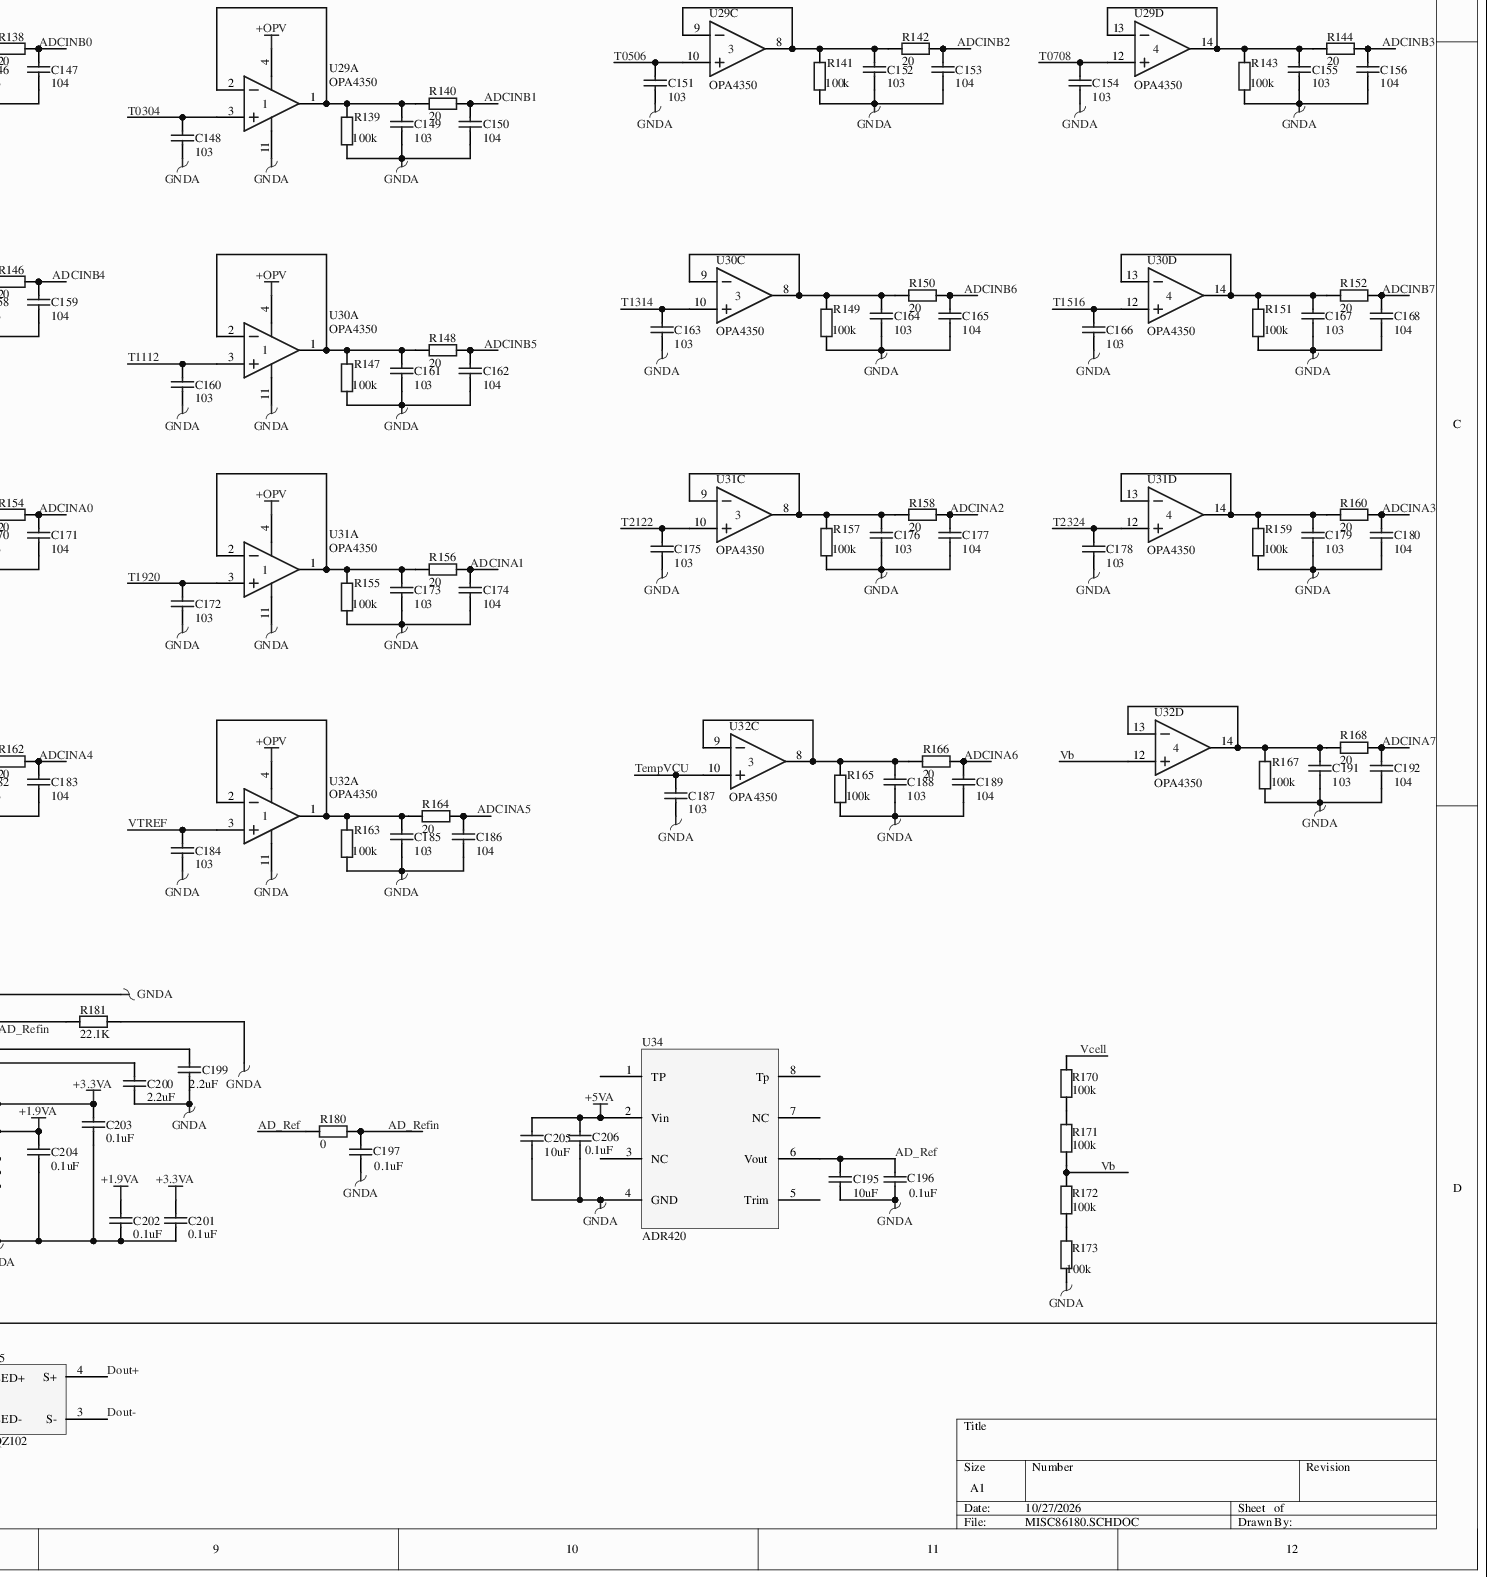
[diagram p0: MISC86180.SCHDOC, bottom right]
# Altium project MISC86180-9.PrjPCB (part 3 of 3)

## Sheet MISC86180.SCHDOC (continued)

### Nets
5VO1+: C9.1 C10.2 C64.2 C65.2 C66.2 C69.2 R23.2 U3.3(+Vout) U13.3(VCC) U15.1(ANODE1) U16.8(Vcc)
5VO1-: C9.2 C10.1 C58.1 C59.1 C60.1 C61.1 C62.1 C63.1 C64.1 C65.1 C66.1 C69.1 DZ1.2 DZ2.2 R20.1 U3.4(-Vout) U13.2(GND) U15.3(CATHODE2) U15.4(ANODE2) U16.5(GND)
+1.9VA: C46.2 C47.2 C48.2 C202.2 C204.2 L3.2 U9.31(VDD1A18) U9.59(VDD2A18)
+1.9VD: C13.1 C14.2 C30.2 C31.2 C32.2 C33.2 C34.2 C35.2 C36.2 C37.2 C38.2 C39.2 C40.2 C41.2 C42.2 L3.1 R3.2 U5.5(OUT) U5.6(OUT) U9.4(VDD(1V8).1) U9.15(VDD(1V8).2) U9.23(VDD(1V8).3) U9.29(VDD(1V8).4) U9.61(VDD(1V8).5) U9.101(VDD(1V8).6) U9.109(VDD(1V8).7) U9.117(VDD(1V8).8) U9.126(VDD(1V8).9) U9.139(VDD(1V8).10) U9.146(VDD(1V8).11) U9.154(VDD(1V8).12) U9.167(VDD(1V8).12)
+3.3VA: C15.1 C16.2 C125.2 C127.2 C201.2 C203.2 JC1.1 R131.1 R133.1 R136.1 U6.4(OUTPUT) U9.34(VDDA2(A3V3)) U9.45(VDDAIO(A3V3))
+3.3VD: C11.1 C12.2 C19.2 C20.2 C21.2 C22.2 C23.2 C24.2 C25.2 C26.2 C27.2 C28.2 C29.2 C68.2 J1.5 R1.1 R2.1 R6.1 R7.1 R8.2 R9.2 R10.2 R11.2 R12.2 R86.1 R88.1 R90.1 R92.1 R94.1 U4.4(OUTPUT) U5.3(IN) U5.4(IN) U8.5(VDD) U9.9(VDDIO(3V3).1) U9.71(VDDIO(3V3).2) U9.84(VDD3VFL.1) U9.93(VDDIO(3V3).3) U9.107(VDDIO(3V3).4) U9.121(VDDIO(3V3).5) U9.143(VDDIO(3V3).6) U9.159(VDDIO(3V3).7) U9.170(VDDIO(3V3).8) U16.1(ANODE1)
+3.3VD2: C17.1 C18.2 C81.1 C82.2 C83.2 C84.2 C85.2 C86.2 C87.2 C88.2 C89.2 C92.2 C93.2 C94.2 C95.2 J3.4 R84.1 R85.1 R95.1 U7.4(OUTPUT) U19.9(VCCIO1) U19.13(VCCINT_(3.3V_or_2.5V)) U19.31(VCCIO1) U19.45(VCCIO1) U19.59(VCCIO2) U19.63(VCCINT_(3.3V_or_2.5V)) U19.80(VCCIO2) U19.94(VCCIO2) U21.23(VCCB) U21.24(VCCB) U22.23(VCCB) U22.24(VCCB) U23.23(VCCB) U23.24(VCCB) U24.23(VCCB) U24.24(VCCB)
+5V: C6.1 C7.2 C57.2 C67.2 C90.2 C91.2 C96.2 C97.2 C98.2 C99.2 R21.2 U2.3(+Vout) U4.2(IN) U7.2(IN) U10.24(VDD) U15.8(Vcc) U20.24(VDD) U21.1(VCCA) U22.1(VCCA) U23.1(VCCA) U24.1(VCCA)
+5VA: C3.1 C4.2 C129.2 C130.2 C131.2 C140.2 C141.2 C142.2 C143.2 C144.2 C205.2 C206.2 U1.3(+Vout) U6.2(IN) U25.16(VCC) U26.16(VCC) U27.16(VCC) U28.16(VCC) U34.2(Vin)
+OPV: C132.2 C133.2 C134.2 C135.2 C136.2 C137.2 C138.2 C139.2 C208.2 C209.2 R136.2 U29.4(V+) U30.4(V+) U31.4(V+) U32.4(V+)
GNDA: C3.2 C4.1 C15.2 C16.1 C46.1 C47.1 C48.1 C100.1 C101.1 C102.1 C103.1 C104.1 C105.1 C106.1 C107.1 C108.1 C109.1 C110.1 C111.1 C112.1 C113.1 C114.1 C115.1 C116.1 C117.1 C118.1 C119.1 C120.1 C121.1 C122.1 C123.1 C124.1 C126.1 C128.1 C129.1 C130.1 C131.1 C132.1 C133.1 C134.1 C135.1 C136.1 C137.1 C138.1 C139.1 C140.1 C141.1 C142.1 C143.1 C144.1 C145.1 C146.1 C147.1 C148.1 C149.1 C150.1 C151.1 C152.1 C153.1 C154.1 C155.1 C156.1 C157.1 C158.1 C159.1 C160.1 C161.1 C162.1 C163.1 C164.1 C165.1 C166.1 C167.1 C168.1 C169.1 C170.1 C171.1 C172.1 C173.1 C174.1 C175.1 C176.1 C177.1 C178.1 C179.1 C180.1 C181.1 C182.1 C183.1 C184.1 C185.1 C186.1 C187.1 C188.1 C189.1 C191.1 C192.1 C195.1 C196.1 C197.1 C199.1 C200.1 C201.1 C202.1 C203.1 C204.1 C205.1 C206.1 C208.1 C209.1 L2.2 R105.1 R106.2 R107.2 R108.2 R109.2 R110.2 R111.2 R112.2 R113.2 R114.2 R115.2 R116.2 R117.2 R118.2 R119.2 R120.2 R121.2 R122.2 R123.2 R124.2 R125.2 R126.2 R127.2 R128.2 R129.2 R130.2 R132.2 R134.2 R137.1 R139.1 R141.1 R143.1 R145.1 R147.1 R149.1 R151.1 R153.1 R155.1 R157.1 R159.1 R161.1 R163.1 R165.1 R167.1 R173.2 R181.2 S1.5(S2_2) S2.5(S2_2) S3.5(S2_2) S4.5(S2_2) S5.5(S2_2) S6.5(S2_2) S7.5(S2_2) S8.5(S2_2) S9.5(S2_2) S10.5(S2_2) S11.5(S2_2) S12.5(S2_2) S13.5(S2_2) S14.5(S2_2) S15.5(S2_2) S16.5(S2_2) S17.5(S2_2) S18.5(S2_2) S19.5(S2_2) S20.5(S2_2) S21.5(S2_2) S22.5(S2_2) S23.5(S2_2) S24.5(S2_2) U1.4(-Vout) U6.1(~{EN}) U6.3(GND) U9.32(VSS1AGND) U9.33(VSSA2(AGND)) U9.43(ADCLO) U9.44(VSSAIO(AGND)) U9.58(VSS2AGND) U25.6(~{EN}) U25.8(GND) U26.6(~{EN}) U26.8(GND) U27.6(~{EN}) U27.8(GND) U28.6(~{EN}) U28.8(GND) U29.11(V-) U30.11(V-) U31.11(V-) U32.11(V-) U34.4(GND)
GNDD: C6.2 C7.1 C11.2 C12.1 C13.2 C14.1 C17.2 C18.1 C19.1 C20.1 C21.1 C22.1 C23.1 C24.1 C25.1 C26.1 C27.1 C28.1 C29.1 C30.1 C31.1 C32.1 C33.1 C34.1 C35.1 C36.1 C37.1 C38.1 C39.1 C40.1 C41.1 C42.1 C52.1 C53.1 C54.1 C55.1 C56.1 C57.1 C67.1 C68.1 C81.2 C82.1 C83.1 C84.1 C85.1 C86.1 C87.1 C88.1 C89.1 C90.1 C91.1 C92.1 C93.1 C94.1 C95.1 C96.1 C97.1 C98.1 C99.1 D1.2(K) D2.2(K) D3.2(K) D4.2(K) D5.2(K) D6.2(K) D7.2(K) D8.2(K) D9.2(K) D10.2(K) J1.4 J1.6 J1.8 J1.10 J1.12 J3.2 J3.10 L2.1 R4.1 R5.1 R14.1 R83.1 R87.2 R89.2 R91.2 R93.2 S1.2(LED1-) S1.4(LED2-) S2.2(LED1-) S2.4(LED2-) S3.2(LED1-) S3.4(LED2-) S4.2(LED1-) S4.4(LED2-) S5.2(LED1-) S5.4(LED2-) S6.2(LED1-) S6.4(LED2-) S7.2(LED1-) S7.4(LED2-) S8.2(LED1-) S8.4(LED2-) S9.2(LED1-) S9.4(LED2-) S10.2(LED1-) S10.4(LED2-) S11.2(LED1-) S11.4(LED2-) S12.2(LED1-) S12.4(LED2-) S13.2(LED1-) S13.4(LED2-) S14.2(LED1-) S14.4(LED2-) S15.2(LED1-) S15.4(LED2-) S16.2(LED1-) S16.4(LED2-) S17.2(LED1-) S17.4(LED2-) S18.2(LED1-) S18.4(LED2-) S19.2(LED1-) S19.4(LED2-) S20.2(LED1-) S20.4(LED2-) S21.2(LED1-) S21.4(LED2-) S22.2(LED1-) S22.4(LED2-) S23.2(LED1-) S23.4(LED2-) S24.2(LED1-) S24.4(LED2-) SW1.2 U2.4(-Vout) U4.1(~{EN}) U4.3(GND) U5.1(GND) U7.1(~{EN}) U7.3(GND) U8.2(GND) U9.3(VSS.1) U9.8(VSS.2) U9.14(VSS.3) U9.22(VSS.4) U9.30(VSS.5) U9.60(VSS.6) U9.70(VSS.7) U9.83(VSS.8) U9.92(VSS.9) U9.103(VSS.10) U9.105(XCLKIN) U9.106(VSS.11) U9.108(VSS.12) U9.118(VSS.13) U9.120(VSS.14) U9.125(VSS.15) U9.140(VSS.16) U9.144(VSS.17) U9.147(VSS.18) U9.155(VSS.19) U9.160(VSS.19) U9.166(VSS.20) U9.171(VSS.21) U10.1(~{OE}1) U10.12(GND) U10.13(~{OE}2) U15.5(GND) U16.3(CATHODE2) U16.4(ANODE2) U19.10(GNDIO) U19.11(GNDINT) U19.32(GNDIO) U19.46(GNDIO) U19.50(IO) U19.60(GNDIO) U19.65(GNDINT) U19.79(GNDIO) U19.93(GNDIO) U20.1(~{OE}1) U20.12(GND) U20.13(~{OE}2) U21.2(DIR) U21.11(GND) U21.12(GND) U21.13(GND) U21.22(~{OE}) U22.2(DIR) U22.11(GND) U22.12(GND) U22.13(GND) U22.22(~{OE}) U23.2(DIR) U23.11(GND) U23.12(GND) U23.13(GND) U23.22(~{OE}) U24.2(DIR) U24.11(GND) U24.12(GND) U24.13(GND) U24.22(~{OE}) U35.1(LED-) Y1.3
12V+: B1.2(CB) C2.1 C5.1 C8.1 U1.1(+Vin) U2.1(+Vin) U3.1(+Vin)
12V-: B1.4(CG) B1.5(CG) B1.6(CG) C2.2 C5.2 C8.2 U1.2(-Vin) U2.2(-Vin) U3.2(-Vin)
12Vin+: F49.2 JC2.26 JC2.34
12Vin-: B1.3(PSG) C1.2 JC2.25 JC2.33 TVS1.1
A1_12: R12.1 U9.169(XA12)
A1_13: R11.1 U9.172(XA13)
A1_14: R10.1 U9.173(XA14)
A1_15: R9.1 U9.174(XA15)
AD_Ref: C195.2 C196.2 R180.2 U34.6(Vout)
AD_Refin: C197.2 R180.1 U9.54(ADCREFIN)
ADCINA0: C171.2 R154.1 U9.42(ADCINA0)
ADCINA1: C174.2 R156.1 U9.41(ADCINA1)
ADCINA2: C177.2 R158.1 U9.40(ADCINA2)
ADCINA3: C180.2 R160.1 U9.39(ADCINA3)
ADCINA4: C183.2 R162.1 U9.38(ADCINA4)
ADCINA5: C186.2 R164.1 U9.37(ADCINA5)
ADCINA6: C189.2 R166.1 U9.36(ADCINA6)
ADCINA7: C192.2 R168.1 U9.35(ADCINA7)
ADCINB0: C147.2 R138.1 U9.46(ADCINB0)
ADCINB1: C150.2 R140.1 U9.47(ADCINB1)
ADCINB2: C153.2 R142.1 U9.48(ADCINB2)
ADCINB3: C156.2 R144.1 U9.49(ADCINB3)
ADCINB4: C159.2 R146.1 U9.50(ADCINB4)
ADCINB5: C162.2 R148.1 U9.51(ADCINB5)
ADCINB6: C165.2 R150.1 U9.52(ADCINB6)
ADCINB7: C168.2 R152.1 U9.53(ADCINB7)
BAT1: F1.1 JC1.24
BAT2: F2.1 F3.1 JC1.32
BAT3: F4.1 F5.1 JC1.25
BAT4: F6.1 F7.1 JC1.33
BAT5: F8.1 F9.1 JC1.26
BAT6: F10.1 F11.1 JC1.34
BAT7: F12.1 F13.1 JC1.27
BAT8: F14.1 F15.1 JC1.35
BAT9: F16.1 F17.1 JC1.28
BAT10: F18.1 F19.1 JC1.36
BAT11: F20.1 F21.1 JC2.3
BAT12: F22.1 F23.1 JC2.13
BAT13: F24.1 F25.1 JC2.4
BAT14: F26.1 F27.1 JC2.14
BAT15: F28.1 F29.1 JC2.5
BAT16: F30.1 F31.1 JC2.15
BAT17: F32.1 F33.1 JC2.6
BAT18: F34.1 F35.1 JC2.16
BAT19: F36.1 F37.1 JC2.7
BAT20: F38.1 F39.1 JC2.17
BAT21: F40.1 F41.1 JC2.8
BAT22: F42.1 F43.1 JC2.18
BAT23: F44.1 F45.1 JC2.9
BAT24: F46.1 F47.1 JC2.19
BAT25: F48.1 JC2.10
CAN1H: C60.2 DZ1.1 JC2.23 JC2.31 R17.2 U11.4
CAN1HIN: C58.2 U11.1 U13.7(CANH)
CAN1L: C61.2 DZ2.1 JC2.22 JC2.30 R18.1 U11.3
CAN1LIN: C59.2 U11.2 U13.6(CANL)
CAN1RX: R22.2 U13.4(R)
CAN1S: JC2.21 JC2.29 R19.2
CAN1TX: R23.1 U13.1(D) U16.7(Vo1)
CANAR: R13.1 R14.2 U10.9(1B4)
CANARR: R13.2 R21.1 U15.7(Vo1)
CANARX: U9.62(GPIO18/SPICLKA/SCITXDB/CANRXA) U10.8(1A4)
CANAT: R24.2 U10.5(1B2)
CANATX: U9.63(GPIO19/SPISTEAn/SCIRXDB/CANTXA) U10.4(1A2)
CI1: U19.69(IO) U20.2(1B1)
CI2: U19.70(IO) U20.10(1B5)
CI3: U19.71(IO) U20.5(1B2)
CI4: U19.72(IO) U20.16(2B2)
CI5: U19.73(IO) U20.6(1B3)
CI6: U19.74(IO) U20.15(2B1)
CI7: U19.75(IO) U20.9(1B4)
CI9: R96.1 U20.23(2B5)
CI10: R97.1 U20.20(2B4)
CO1: U19.66(IO) U22.16(B6)
CO2: U19.64(IO/GCLK3) U22.17(B5)
CO3: U19.62(IO/GCLK2) U22.18(B4)
CO4: U19.61(IO) U22.19(B3)
CO5: U19.57(IO) U22.21(B1)
CO6: U19.58(IO) U22.20(B2)
CO7: U19.51(IO) U21.14(B8)
CO8: U19.52(IO) U21.15(B7)
CO9: U19.53(IO) U21.16(B6)
CO10: U19.54(IO) U21.17(B5)
CO11: U19.55(IO) U21.18(B4)
CO12: U19.56(IO) U21.19(B3)
CO13: U19.7(IO) U23.19(B3)
CO14: U19.8(IO) U23.18(B4)
CO15: U19.12(IO/GCLK0) U23.17(B5)
CO16: U19.14(IO/GCLK1) U23.16(B6)
CO17: U19.15(IO) U23.15(B7)
CO18: U19.16(IO) U23.14(B8)
CO19: U19.6(IO) U24.19(B3)
CO20: U19.5(IO) U24.18(B4)
CO21: U19.4(IO) U24.17(B5)
CO22: U19.3(IO) U24.16(B6)
CO23: U19.2(IO) U24.15(B7)
CO24: U19.1(IO) U24.14(B8)
CO25: U19.67(IO) U22.15(B7)
CO26: U19.68(IO) U22.14(B8)
CT1: R33.2 R34.2 U22.8(A6)
CT2: R35.2 R36.2 U22.7(A5)
CT3: R37.2 R38.2 U22.6(A4)
CT4: R41.2 R42.2 U22.5(A3)
CT5: R43.2 R44.2 U22.3(A1)
CT6: R45.2 R46.2 U22.4(A2)
CT7: R47.2 R48.2 U21.10(A8)
CT8: R49.2 R50.2 U21.9(A7)
CT9: R51.2 R52.2 U21.8(A6)
CT10: R53.2 R54.2 U21.7(A5)
CT11: R55.2 R56.2 U21.6(A4)
CT12: R57.2 R58.2 U21.5(A3)
CT13: R59.2 R60.2 U23.5(A3)
CT14: R61.2 R62.2 U23.6(A4)
CT15: R63.2 R64.2 U23.7(A5)
CT16: R65.2 R66.2 U23.8(A6)
CT17: R67.2 R68.2 U23.9(A7)
CT18: R69.2 R70.2 U23.10(A8)
CT19: R71.2 R72.2 U24.5(A3)
CT20: R73.2 R74.2 U24.6(A4)
CT21: R75.2 R76.2 U24.7(A5)
CT22: R77.2 R78.2 U24.8(A6)
CT23: R79.2 R80.2 U24.9(A7)
CT24: R81.2 R82.2 U24.10(A8)
CT25: L1.1 U22.10(A8)
CT26: R104.2 U22.9(A7)
CTCK: J3.1 R83.2 U19.24(TCK)
CTDI: J3.9 R85.2 U19.23(TDI)
CTDO: J3.3 U19.25(TDO)
CTMS: J3.5 R84.2 U19.22(TMS)
CTOUT25: L1.2 R105.2 U25.9(C) U25.10(B) U25.11(A) U26.9(C) U26.10(B) U26.11(A) U27.9(C) U27.10(B) U27.11(A) U28.9(C) U28.10(B) U28.11(A)
Dout+: JC2.24 U35.4(S+)
Dout-: JC2.32 U35.3(S-)
EMU0: C53.2 J1.13 R6.2 U9.85(EMU0)
EMU1: C54.2 J1.14 R7.2 U9.86(EMU1)
GPIO0: U9.5(GPIO0/EPWM1A) U20.3(1A1)
GPIO1: U9.6(GPIO1/EPWM1B/ECAP6/MFSRB) U20.11(1A5)
GPIO2: U9.7(GPIO2/EPWM2A) U20.4(1A2)
GPIO3: U9.10(GPIO3/EPWM2B/ECAP5/MCLKRB) U20.17(2A2)
GPIO4: U9.11(GPIO4/EPWM3A) U20.7(1A3)
GPIO5: U9.12(GPIO5/EPWM3B/MFSRA/ECAP1) U20.14(2A1)
GPIO6: U9.13(GPIO6/EPWM4A/EPWMSYNCI/EPWMSYNCO) U20.8(1A4)
GPIO8: U9.17(GPIO8/EPWM5A/CANTXB/ADCSOCAOn) U20.22(2A5)
GPIO9: U9.18(GPIO9/EPWM5B/SCITXDB/ECAP3) U20.21(2A4)
GPIO10: R86.2 R87.1 U9.19(GPIO10/EPWM6A/CANRXB/ADCSOCBOn)
GPIO11: R88.2 R89.1 U9.20(GPIO11/EPWM6B/SCIRXDB/ECAP4)
GPIO12: R90.2 R91.1 U9.21(GPIO12/TZ1n/CANTXB/MDXB)
GPIO13: R92.2 R93.1 U9.24(GPIO13/TZ2n/CANRXB/MDRB)
LED1: R98.1 U19.76(IO)
LED2: R99.1 U19.81(IO)
LED3: R100.1 U19.82(IO)
LED4: R101.1 U19.88(IO)
LED5: R102.1 U19.89(IO)
LED6: R103.1 U19.97(IO)
~{MR}: SW1.1 U8.3(~{MR})
~{PG}: R1.2 U4.5(FB/~{PG}) U5.2(~{EN})
~{RESET}: R2.2 U8.1(~{RESE}T) U9.80(~{XRS})
T0102: C145.2 U25.14(X) U29.5(IN+)
T0304: C148.2 U25.15(Y) U29.3(IN+)
T0506: C151.2 U25.4(Z) U29.10(IN+)
T0708: C154.2 U28.14(X) U29.12(IN+)
T0910: C157.2 U28.15(Y) U30.5(IN+)
T1112: C160.2 U28.4(Z) U30.3(IN+)
T1314: C163.2 U27.15(Y) U30.10(IN+)
T1516: C166.2 U27.4(Z) U30.12(IN+)
T1718: C169.2 U27.14(X) U31.5(IN+)
T1920: C172.2 U26.14(X) U31.3(IN+)
T2122: C175.2 U26.15(Y) U31.10(IN+)
T2324: C178.2 U26.4(Z) U31.12(IN+)
~{TRST}: C52.2 J1.2 R5.2 U9.78(~{TRST})
TCK: J1.9 J1.11 U9.87(TCK)
TDI: J1.3 U9.76(TDI)
TDO: J1.7 U9.77(TDO)
Temp1: C100.2 JC1.11 R106.1 U25.12(X0)
Temp2: C101.2 JC1.2 R107.1 U25.13(X1)
Temp3: C102.2 JC1.12 R108.1 U25.2(Y0)
Temp4: C103.2 JC1.3 R109.1 U25.1(Y1)
Temp5: C104.2 JC1.13 R110.1 U25.5(Z0)
Temp6: C105.2 JC1.4 R111.1 U25.3(Z1)
Temp7: C106.2 JC1.14 R112.1 U28.12(X0)
Temp8: C107.2 JC1.5 R113.1 U28.13(X1)
Temp9: C108.2 JC1.15 R114.1 U28.2(Y0)
Temp10: C109.2 JC1.6 R115.1 U28.1(Y1)
Temp11: C110.2 JC1.16 R116.1 U28.5(Z0)
Temp12: C111.2 JC1.7 R117.1 U28.3(Z1)
Temp13: C112.2 JC1.17 R118.1 U27.2(Y0)
Temp14: C113.2 JC1.8 R119.1 U27.1(Y1)
Temp15: C114.2 JC1.18 R120.1 U27.5(Z0)
Temp16: C115.2 JC1.9 R121.1 U27.3(Z1)
Temp17: C116.2 JC1.19 R122.1 U27.12(X0)
Temp18: C117.2 JC1.10 R123.1 U27.13(X1)
Temp19: C118.2 JC1.20 R124.1 U26.12(X0)
Temp20: C119.2 JC1.21 R125.1 U26.13(X1)
Temp21: C120.2 JC1.29 R126.1 U26.2(Y0)
Temp22: C121.2 JC1.22 R127.1 U26.1(Y1)
Temp23: C122.2 JC1.30 R128.1 U26.5(Z0)
Temp24: C123.2 JC1.23 R129.1 U26.3(Z1)
Temp25: C124.2 C181.2 JC1.31 R130.1 U32.5(IN+)
TempVCU: C127.1 C128.2 C187.2 R133.2 R134.1 U32.10(IN+)
TMS: J1.1 U9.79(TMS)
Vb: R171.2 R172.1 U32.12(IN+)
Vcell: R170.1 S1.7(S1_2) S2.7(S1_2) S3.7(S1_2) S4.7(S1_2) S5.7(S1_2) S6.7(S1_2) S7.7(S1_2) S8.7(S1_2) S9.7(S1_2) S10.7(S1_2) S11.7(S1_2) S12.7(S1_2) S13.7(S1_2) S14.7(S1_2) S15.7(S1_2) S16.7(S1_2) S17.7(S1_2) S18.7(S1_2) S19.7(S1_2) S20.7(S1_2) S21.7(S1_2) S22.7(S1_2) S23.7(S1_2) S24.7(S1_2)
VTREF: C125.1 C126.2 C184.2 R131.2 R132.1 U32.3(IN+)
NetB1_1: B1.1(B) C1.1 F49.1 TVS1.2
NetC55_2: C55.2 U9.102(X2) Y1.1
NetC56_2: C56.2 U9.104(X1) Y1.2
NetC62_2: C62.2 R17.1 R18.2
NetC63_2: C63.2 R19.1
NetC146_2: C146.2 R137.2 R138.2 U29.6(IN-) U29.7(OUT)
NetC149_2: C149.2 R139.2 R140.2 U29.1(OUT) U29.2(IN-)
NetC152_2: C152.2 R141.2 R142.2 U29.8(OUT) U29.9(IN-)
NetC155_2: C155.2 R143.2 R144.2 U29.13(IN-) U29.14(OUT)
NetC158_2: C158.2 R145.2 R146.2 U30.6(IN-) U30.7(OUT)
NetC161_2: C161.2 R147.2 R148.2 U30.1(OUT) U30.2(IN-)
NetC164_2: C164.2 R149.2 R150.2 U30.8(OUT) U30.9(IN-)
NetC167_2: C167.2 R151.2 R152.2 U30.13(IN-) U30.14(OUT)
NetC170_2: C170.2 R153.2 R154.2 U31.6(IN-) U31.7(OUT)
NetC173_2: C173.2 R155.2 R156.2 U31.1(OUT) U31.2(IN-)
NetC176_2: C176.2 R157.2 R158.2 U31.8(OUT) U31.9(IN-)
NetC179_2: C179.2 R159.2 R160.2 U31.13(IN-) U31.14(OUT)
NetC182_2: C182.2 R161.2 R162.2 U32.6(IN-) U32.7(OUT)
NetC185_2: C185.2 R163.2 R164.2 U32.1(OUT) U32.2(IN-)
NetC188_2: C188.2 R165.2 R166.2 U32.8(OUT) U32.9(IN-)
NetC191_2: C191.2 R167.2 R168.2 U32.13(IN-) U32.14(OUT)
NetC199_2: C199.2 U9.56(ADCREFP)
NetC200_2: C200.2 U9.55(ADCREFM)
NetD1_1: D1.1(A) R94.2
NetD2_1: D2.1(A) R95.2
NetD3_1: D3.1(A) R96.2
NetD4_1: D4.1(A) R97.2
NetD5_1: D5.1(A) R98.2
NetD6_1: D6.1(A) R99.2
NetD7_1: D7.1(A) R100.2
NetD8_1: D8.1(A) R101.2
NetD9_1: D9.1(A) R102.2
NetD10_1: D10.1(A) R103.2
NetF1_2: F1.2 S1.8(S1_1)
NetF2_2: F2.2 S1.6(S2_1)
NetF3_2: F3.2 S2.8(S1_1)
NetF4_2: F4.2 S2.6(S2_1)
NetF5_2: F5.2 S3.8(S1_1)
NetF6_2: F6.2 S3.6(S2_1)
NetF7_2: F7.2 S4.8(S1_1)
NetF8_2: F8.2 S4.6(S2_1)
NetF9_2: F9.2 S5.8(S1_1)
NetF10_2: F10.2 S5.6(S2_1)
NetF11_2: F11.2 S6.8(S1_1)
NetF12_2: F12.2 S6.6(S2_1)
NetF13_2: F13.2 S7.8(S1_1)
NetF14_2: F14.2 S7.6(S2_1)
NetF15_2: F15.2 S8.8(S1_1)
NetF16_2: F16.2 S8.6(S2_1)
NetF17_2: F17.2 S9.8(S1_1)
NetF18_2: F18.2 S9.6(S2_1)
NetF19_2: F19.2 S10.8(S1_1)
NetF20_2: F20.2 S10.6(S2_1)
NetF21_2: F21.2 S11.8(S1_1)
NetF22_2: F22.2 S11.6(S2_1)
NetF23_2: F23.2 S12.8(S1_1)
NetF24_2: F24.2 S12.6(S2_1)
NetF25_2: F25.2 S13.8(S1_1)
NetF26_2: F26.2 S13.6(S2_1)
NetF27_2: F27.2 S14.8(S1_1)
NetF28_2: F28.2 S14.6(S2_1)
NetF29_2: F29.2 S15.8(S1_1)
NetF30_2: F30.2 S15.6(S2_1)
NetF31_2: F31.2 S16.8(S1_1)
NetF32_2: F32.2 S16.6(S2_1)
NetF33_2: F33.2 S17.8(S1_1)
NetF34_2: F34.2 S17.6(S2_1)
NetF35_2: F35.2 S18.8(S1_1)
NetF36_2: F36.2 S18.6(S2_1)
NetF37_2: F37.2 S19.8(S1_1)
NetF38_2: F38.2 S19.6(S2_1)
NetF39_2: F39.2 S20.8(S1_1)
NetF40_2: F40.2 S20.6(S2_1)
NetF41_2: F41.2 S21.8(S1_1)
NetF42_2: F42.2 S21.6(S2_1)
NetF43_2: F43.2 S22.8(S1_1)
NetF44_2: F44.2 S22.6(S2_1)
NetF45_2: F45.2 S23.8(S1_1)
NetF46_2: F46.2 S23.6(S2_1)
NetF47_2: F47.2 S24.8(S1_1)
NetF48_2: F48.2 S24.6(S2_1)
NetJ2_1: J2.1 U9.99(GPIO57/SPISTEAn/XD22)
NetJ2_2: J2.2 U9.98(GPIO56/SPICLKA/XD23)
NetJ2_3: J2.3 U9.97(GPIO55/SPISOMIA/XD24)
NetJ2_4: J2.4 U9.96(GPIO54/SPISIMOA/XD25)
NetR3_1: R3.1 R4.2 U5.7(FB/NC)
NetR8_1: R8.1 U9.142(XREADY)
NetR20_2: R20.2 U13.8(RS)
NetR22_1: R22.1 U15.2(CATHODE1)
NetR24_1: R24.1 U16.2(CATHODE1)
NetR33_1: R33.1 S1.1(LED1+)
NetR34_1: R34.1 S1.3(LED2+)
NetR35_1: R35.1 S2.1(LED1+)
NetR36_1: R36.1 S2.3(LED2+)
NetR37_1: R37.1 S3.1(LED1+)
NetR38_1: R38.1 S3.3(LED2+)
NetR41_1: R41.1 S4.1(LED1+)
NetR42_1: R42.1 S4.3(LED2+)
NetR43_1: R43.1 S5.1(LED1+)
NetR44_1: R44.1 S5.3(LED2+)
NetR45_1: R45.1 S6.1(LED1+)
NetR46_1: R46.1 S6.3(LED2+)
NetR47_1: R47.1 S7.1(LED1+)
NetR48_1: R48.1 S7.3(LED2+)
NetR49_1: R49.1 S8.1(LED1+)
NetR50_1: R50.1 S8.3(LED2+)
NetR51_1: R51.1 S9.1(LED1+)
NetR52_1: R52.1 S9.3(LED2+)
NetR53_1: R53.1 S10.1(LED1+)
NetR54_1: R54.1 S10.3(LED2+)
NetR55_1: R55.1 S11.1(LED1+)
NetR56_1: R56.1 S11.3(LED2+)
NetR57_1: R57.1 S12.1(LED1+)
NetR58_1: R58.1 S12.3(LED2+)
NetR59_1: R59.1 S13.1(LED1+)
NetR60_1: R60.1 S13.3(LED2+)
NetR61_1: R61.1 S14.1(LED1+)
NetR62_1: R62.1 S14.3(LED2+)
NetR63_1: R63.1 S15.1(LED1+)
NetR64_1: R64.1 S15.3(LED2+)
NetR65_1: R65.1 S16.1(LED1+)
NetR66_1: R66.1 S16.3(LED2+)
NetR67_1: R67.1 S17.1(LED1+)
NetR68_1: R68.1 S17.3(LED2+)
NetR69_1: R69.1 S18.1(LED1+)
NetR70_1: R70.1 S18.3(LED2+)
NetR71_1: R71.1 S19.1(LED1+)
NetR72_1: R72.1 S19.3(LED2+)
NetR73_1: R73.1 S20.1(LED1+)
NetR74_1: R74.1 S20.3(LED2+)
NetR75_1: R75.1 S21.1(LED1+)
NetR76_1: R76.1 S21.3(LED2+)
NetR77_1: R77.1 S22.1(LED1+)
NetR78_1: R78.1 S22.3(LED2+)
NetR79_1: R79.1 S23.1(LED1+)
NetR80_1: R80.1 S23.3(LED2+)
NetR81_1: R81.1 S24.1(LED1+)
NetR82_1: R82.1 S24.3(LED2+)
NetR104_1: R104.1 U35.2(LED+)
NetR170_2: R170.2 R171.1
NetR172_2: R172.2 R173.1
NetR181_1: R181.1 U9.57(ADCRESEXT)

Not connected (* = marked no-connect by the designer): J3 6 7 8; JC2 20; U5 8(PG)*; U6 5(FB/~{PG}); U7 5(FB/~{PG}); U8 4(WDI)*; U9 1(XA18)* 2(XA19)* 16(GPIO7/EPWM4B/MCLKRA/ECAP2) 25(~{XHOLD})* 26(~{XHOLDA})* 27(GPIO16/SPISIMOA/CANTXB/TZ5n)* 28(GPIO17/SPISOMIA/CANRXB/TZ6n)* 64(GPIO20/EQEP1A/MDXA/CANTXB)* 65(GPIO21/EQEP1B/MDRA/CANRXB)* 66(GPIO22/EQEP1S/MCLKXA/SCITXDB)* 67(GPIO23/EQEP1I/MFSXA/SCIRXDB)* 68(GPIO24/ECAP1/EQEP2A/MDXB)* 69(GPIO25/ECAP2/EQEP2B/MDRB)* 72(GPIO26/ECAP3/EQEP2I/MCLKXB)* 73(GPIO27/ECAP4/EQEP2S/MFSXB)* 74(GPIO32/SDAA/EPWMSYNCI/ADCSOCAOn)* 75(GPIO33/SCLA/EPWMSYNCO/ADCSOCBOn)* 81((NC)_TEST1)* 82((NC)_TEST2)* 88(GPIO48/ECAP5/XD31)* 89(GPIO49/ECAP6/XD30)* 90(GPIO50/EQEP1A/XD29)* 91(GPIO51/EQEP1B/XD28)* 94(GPIO52/EQEP1S/XD27)* 95(GPIO53/EQEP1I/XD26)* 100(GPIO58/MCLKRA/XD21)* 110(GPIO59/MFSRA/XD20)* 111(GPIO60/MCLKRB/XD19)* 112(GPIO61/MFSRB/XD18)* 113(GPIO62/SCIRXDC/XD17)* 114(GPIO63/SCITXDC/XD16)* 115(XD15)* 116(XD14)* 119(XD13)* 122(XD12)* 123(XD11)* 124(XD10)* 127(XD9)* 128(XD8)* 129(XD7)* 130(XD6)* 131(XD5)* 132(XD4)* 133(XD3)* 134(XD2)* 135(XD1)* 136(XD0)* 137(~{XWE0})* 138(XCLKOUT)* 141(~{XZCS6})* 145(~{XZCS0})* 148(XR~{W})* 149(~{XRD})* 150(~{XZCS7})* 151(XA0/~{XWE1})* 152(XA1)* 153(XA2)* 156(XA3)* 157(XA4)* 158(XA5)* 161(XA6)* 162(XA7)* 163(XA8)* 164(XA9)* 165(XA10)* 168(XA11)* 175(XA16)* 176(XA17)*; U10 2(1B1) 3(1A1) 6(1B3) 7(1A3) 10(1B5) 11(1A5) 14(2A1) 15(2B1) 16(2B2) 17(2A2) 18(2A3) 19(2B3) 20(2B4) 21(2A4) 22(2A5) 23(2B5); U13 5(VREF)*; U15 6(Vo2); U16 6(Vo2); U19 17(IO) 18(IO) 19(IO) 20(IO) 21(IO) 26(IO) 27(IO) 28(IO) 29(IO) 30(IO) 33(IO) 34(IO) 35(IO) 36(IO) 37(IO) 38(IO) 39(IO) 40(IO) 41(IO) 42(IO) 43(IO/DEV_OE) 44(IO/DEV_CLRn) 47(IO) 48(IO) 49(IO) 77(IO) 78(IO) 83(IO) 84(IO) 85(IO) 86(IO) 87(IO) 90(IO) 91(IO) 92(IO) 95(IO) 96(IO) 98(IO) 99(IO) 100(IO); U20 18(2A3) 19(2B3); U21 3(A1) 4(A2) 20(B2) 21(B1); U23 3(A1) 4(A2) 20(B2) 21(B1); U24 3(A1) 4(A2) 20(B2) 21(B1); U25 7(VEE); U26 7(VEE); U27 7(VEE); U28 7(VEE); U34 1(TP) 3(NC) 5(Trim) 7(NC) 8(Tp)

### Notes on the sheet
- (near J1) JTAG
- (near F49) POWER
- (near U9) XINTF
- CAN
- EXTERN
- AD
- (near U25) TEMP
- SWITCH
- (near U19) GPIO
- Dout

### Library data of the parts
C1-C3 C5 C6 C8 C9 C11 C13 C15 C17 C81 = Cap Pol3: Polarized Capacitor (Surface Mount); Published: 8-Jun-2000; Revision: July-2002: Re-released for DXP Platform.; Publisher: Altium Limited
C4 C7 C10 C12 C14 C16 C18-C42 C46-C48 C52-C69 C82-C189 C191 C192 C195-C197 C199-C206 C208 C209 = Cap: Capacitor; Published: 8-Jun-2000; Publisher: Altium Limited
  C4 C7 C10 C12 C14 C16 C18-C42 C46-C48 C52-C69 C82-C89 C91-C99 C129-C135 C143 C145-C189 C191 C192 C195 C199-C205 C208: Revision: July-2002: Re-released for DXP Platform.
  C90 C100-C128: Revision: July-2002: Re-released for DXP Platform.; value: value
  C136-C142 C144 C196 C197 C206 C209: LatestRevisionDate: 17-Jul-2002; LatestRevisionNote: Re-released for DXP Platform.
D1-D10 = LED1: Typical YELLOW GaAs LED; Published: 8-Jun-2000; Revision: July-2002: Re-released for DXP Platform.; Publisher: Altium Limited
  D1 D2: Value: RED
  D3 D4: Value: GREEN
  D5-D9: Value: BLUE
DZ1 DZ2 = AK1B
F1-F48 R1-R14 R17-R24 R33-R38 R41-R134 R136-R168 R170-R173 R180 R181 = Res2: Resistor; Published: 8-Jun-2000; Revision: July-2002: Re-released for DXP Platform.; Publisher: Altium Limited
F49 = FUSE1: Fuse
J1 = Header 7X2A: Header, 7-Pin, Dual row; Revision: 17-Jul-2002: Re-released for DXP Platform.; Publisher: Altium Limited
J2 = Header 4: Header, 4-Pin; LatestRevisionDate: 17-Jul-2002; LatestRevisionNote: Re-released for DXP Platform.; Publisher: Altium Limited
J3 = Header 5X2: Header, 5-Pin, Dual row; LatestRevisionDate: 17-Jul-2002; LatestRevisionNote: Re-released for DXP Platform.; Publisher: Altium Limited
SW1 = SW-PB: Switch; Published: 24-Mar-1999; Revision: July-2002: Re-released for DXP Platform.; Publisher: Altium Limited
TVS1 = diode2
U1-U3 = DCDC
U10 U20 = SN74CBTD3384DBLE: 10-Bit FET Bus Switch with Level Shifting; Package Information: Latest Revision: May-1999; Code - JEDEC: MO-150-AG; Published: 8-Jun-2000; Revision: 17-Jul-2002: Re-released for DXP Platform.; Datasheet: Latest Revision: Nov-1998; Package Reference: DB024; Publisher: Altium Limited
U19 = EPM240T100C5N: MAX II 2.5/3.3V CPLD, 80 I/Os, 100-Pin Plastic TQFP, Pb-Free, Commercial Temperature, Speed Grade 5; PackageDocument: ver13.0, May-2005; Note: Each set of VCCIO pins can be connected to 3.3V, 2.5V, 1.8V, or 1.5V.; Published: 4-Mar-2005; LatestRevisionDate: 4-Mar-2005; LatestRevisionNote: Stylized 3D Model Added.; DatasheetDocument: ver1.1, Jun-2004; PackageReference: TQFP100; Code_JEDEC: MS-026-AED; Code_IPC: SQFP14X14-100; ComponentLink1Description: Manufacturer Link; ComponentLink1URL: http://www.altera.com/products/devices/cpld/max2/mx2-index.jsp; ComponentLink2Description: Handbook; ComponentLink2URL: http://www.altera.com/literature/hb/max2/max2_mii5v1.pdf; ComponentLink3Description: Pinout Specification; ComponentLink3URL: http://www.altera.com/literature/dp/max2/epm240.pdf; ComponentLink4Description: Packaging Specification; ComponentLink5Description: Lead-Free Devices; Publisher: Altium Limited
U21-U24 = SN74LVC4245PW: Octal Bus Transceiver and 3.3-V to 5-V Shifter with 3-State Outputs; Published: 8-Jun-2000; LatestRevisionDate: 4-Mar-2005; LatestRevisionNote: Stylized 3D Model Added.; DatasheetDocument: Jan-1997; PackageDocument: Feb-1999; PackageReference: PW024; ComponentLink1Description: Manufacturer Link; Publisher: Altium Limited
U25-U28 = M74HC4053M1R: Analog Multiplexer/Demultiplexer Triple 2-Channel; Published: 8-Jun-2000; LatestRevisionDate: 6-Jun-2005; LatestRevisionNote: Stylized 3D Model Added.; DatasheetDocument: Oct-1993; PackageDocument: May-1998; PackageReference: SO16; ComponentLink1Description: Manufacturer Link; Publisher: Altium Limited
U29-U32 = LM324D: Quad Low-Power Operational Amplifier; PackageDocument: 1991; Published: 17-Jul-2002; LatestRevisionDate: 6-Jun-2005; LatestRevisionNote: Stylized 3D Model Added.; DatasheetDocument: 1988; PackageReference: 751A-02; ComponentLink1Description: Manufacturer Link; Publisher: Altium Limited
U34 = ADR421
U35 = AQZ
Y1 = CRYSTAL
L1-L3 = Inductor: Published: 8-Jun-2000; Revision: July-2002: Re-released for DXP Platform.; Publisher: Altium Limited
U9 = TMS320F283XXPGF_23: Right: *; Bottom: *; Part #: *